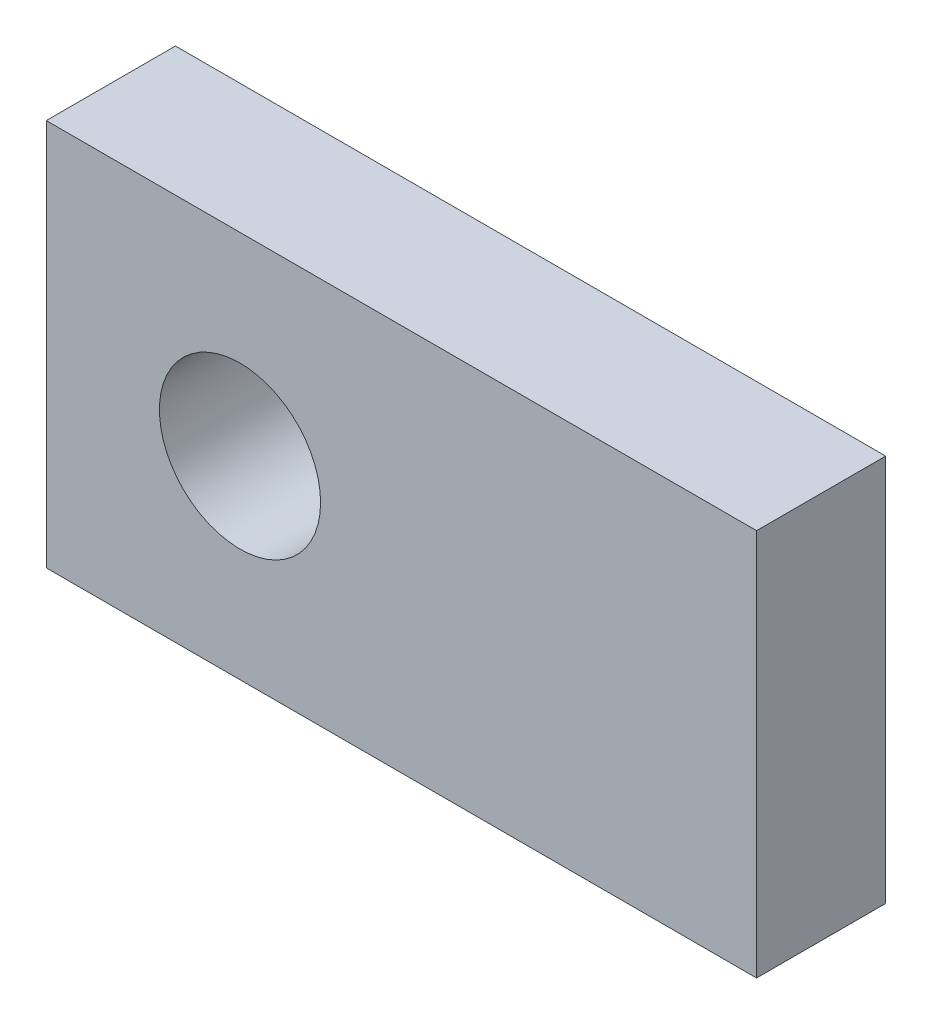
SolidWorks part; units mm, degrees
ref_plane "Front Plane" through (0, 0, 0) normal (0, 0, 1) x (1, 0, 0)
ref_plane "Top Plane" through (0, 0, 0) normal (0, 1, 0) x (1, 0, 0)
ref_plane "Right Plane" through (0, 0, 0) normal (1, 0, 0) x (0, 0, -1)
sketch "Sketch1" plane through (0, 0, 0) normal (0, 0, 1) x (1, 0, 0)
  line L1 (0, 0) -> (34.925, 0)
  line L2 (0, 0) -> (0, 19.05)
  line L3 (0, 19.05) -> (34.925, 19.05)
  line L4 (34.925, 0) -> (34.925, 19.05)
  circle A0 centre (9.525, 9.525) radius 3.9624
  dimension "D1" = 7.9248
  dimension "D2" = 9.525
  dimension "D3" = 9.525
  dimension "D4" = 34.925
  dimension "D5" = 19.05
extrude "Boss-Extrude1" add sketch "Sketch1" along normal blind 6.35
